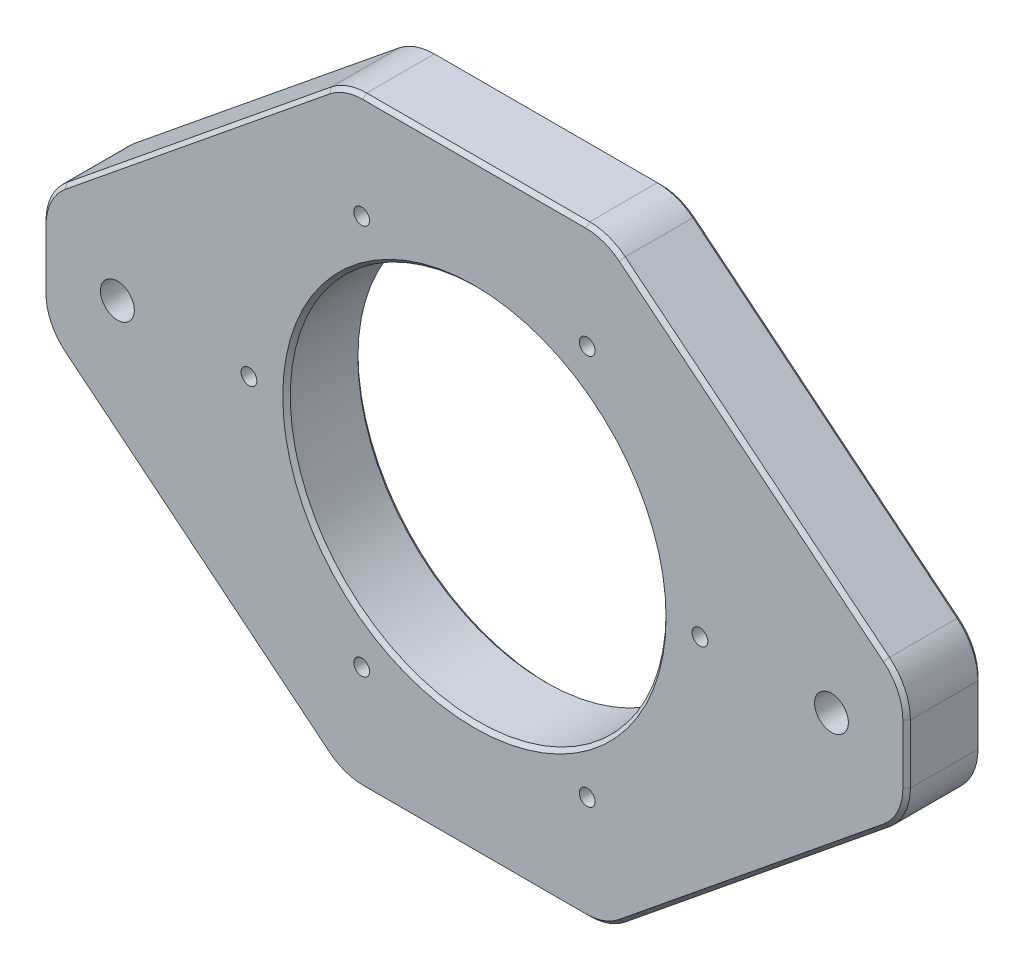
SolidWorks part; units mm, degrees
material "P20"
ref_plane "Front Plane" through (0, 0, 0) normal (0, 0, 1) x (1, 0, 0)
ref_plane "Top Plane" through (0, 0, 0) normal (0, 1, 0) x (1, 0, 0)
ref_plane "Right Plane" through (0, 0, 0) normal (1, 0, 0) x (0, 0, -1)
sketch "Sketch1" plane through (0, 0, 0) normal (0, 0, 1) x (1, 0, 0)
  line L1 (-115, -80) -> (115, -80)
  line L2 (-115, -80) -> (-115, 80)
  line L3 (-115, 80) -> (115, 80)
  line L4 (115, -80) -> (115, 80)
  line L5 (-115, -80) -> (115, 80) construction
  line L6 (-115, 80) -> (115, -80) construction
  circle A0 centre (0, 0) radius 115 construction
  point P0 (0, 0)
  dimension "D3" = 230
  dimension "D1" = 230
  dimension "D2" = 160
extrude "Boss-Extrude1" add sketch "Sketch1" along normal blind 20
sketch "Sketch4" plane through (0, 0, 20) normal (0, 0, 1) x (1, 0, 0)
  circle A0 centre (0, 0) radius 50
  dimension "D1" = 100
extrude "Cut-Extrude3" cut sketch "Sketch4" against normal blind 109
sketch "Sketch5" plane through (0, 0, 0) normal (0, 0, 1) x (1, 0, 0)
  line L0 (0, 0) -> (-95, 0) construction
  line L1 (0, 0) -> (95, 0) construction
  line L2 (0, 0) -> (0, 179.4506) construction
  circle A0 centre (-95, 0) radius 10.25
  circle A1 centre (95, 0) radius 10.25
  dimension "D1" = 20.5
  dimension "D2" = 190
extrude "Cut-Extrude4" cut sketch "Sketch5" along normal blind 6
hole_wizard "M8 Clearance Hole1" positions "Sketch6" profile "Sketch8" hole size "M8" standard "GB" end condition through all
sketch "Sketch6" plane through (0, 0, 20) normal (0, 0, 1) x (1, 0, 0)
  point P0 (-95, 0)
  point P2 (95, 0)
sketch "Sketch8" plane through (-95, 0, 20) normal (1, 0, 0) x (0, -1, 0)
  line L0 (0, 0) -> (0, 20)
  line L1 (0, 20) -> (4.5, 20)
  line L2 (4.5, 20) -> (4.5, 0)
  line L5 (4.5, 0) -> (0, 0)
  line L11 (0, -6.35) -> (0, 107.95) construction
  dimension "通孔孔直径" = 9
  dimension "通孔孔深度" = 20
chamfer "Chamfer2" distance 1 angle 45 2 edges at (50, 0, 20) (-50, 0, 0)
sketch "Sketch10" plane through (0, 0, 20) normal (0, 0, 1) x (1, 0, 0)
  line L0 (-115, 80) -> (-35, 80)
  line L1 (115, 80) -> (-115, 80) construction
  line L2 (-35, 80) -> (-115, 15)
  line L3 (-115, 80) -> (-115, -80) construction
  line L4 (-115, 15) -> (-115, 80)
  line L5 (35, 80) -> (115, 80)
  line L6 (115, 80) -> (115, 15)
  line L7 (115, -80) -> (115, 80) construction
  line L8 (115, 15) -> (35, 80)
  line L9 (-115, -15) -> (-35, -80)
  line L10 (-115, -80) -> (115, -80) construction
  line L11 (-35, -80) -> (-115, -80)
  line L12 (-115, -80) -> (-115, -15)
  line L13 (35, -80) -> (115, -80)
  line L14 (115, -80) -> (115, -15)
  line L15 (115, -15) -> (35, -80)
  line L16 (0, 80) -> (0, -80) construction
  line L17 (-115, 0) -> (115, 0) construction
  dimension "D1" = 80
  dimension "D2" = 65
extrude "Cut-Extrude6" cut sketch "Sketch10" against normal blind 214
fillet "Fillet1" radius 15 8 edges at (-115, 15, 10) (-35, 80, 10) (35, 80, 10) (115, 15, 10) (115, -15, 10) (35, -80, 10) (-35, -80, 10) (-115, -15, 10)
chamfer "Chamfer3" distance 1 angle 45 32 edges at (115, 0, 0) (113.5441, 14.307, 0) (113.5441, -14.307, 0) (74.2961, 48.0719, 0) (74.2961, -48.0719, 0) (34.6931, 79.1355, 0) (34.6931, -79.1355, 0) (0, 80, 0) (0, -80, 0) (-34.6931, 79.1355, 0) (-34.6931, -79.1355, 0) (-74.2961, 48.0719, 0) (-74.2961, -48.0719, 0) (-113.5441, 14.307, 0) (-113.5441, -14.307, 0) (-115, 0, 0) (74.2961, -48.0719, 20) (34.6931, -79.1355, 20) (113.5441, -14.307, 20) (0, -80, 20) (115, 0, 20) (-34.6931, -79.1355, 20) (113.5441, 14.307, 20) (-74.2961, -48.0719, 20) (74.2961, 48.0719, 20) (-113.5441, -14.307, 20) (34.6931, 79.1355, 20) (-115, 0, 20) (0, 80, 20) (-113.5441, 14.307, 20) (-34.6931, 79.1355, 20) (-74.2961, 48.0719, 20)
chamfer "Chamfer4" distance 1 angle 45 2 edges at (105.25, 0, 0) (-84.75, 0, 0)
hole_wizard "M5 Tapped Hole1" positions "Sketch11" profile "Sketch12" tap size "M5" standard "GB" end condition through all
sketch "Sketch11" plane through (0, 0, 20) normal (0, 0, 1) x (1, 0, 0)
  point P0 (-30, 51.9615)
  point P3 (-60, 0)
  point P6 (-30, -51.9615)
  point P9 (30, -51.9615)
  point P12 (60, 0)
  point P15 (30, 51.9615)
sketch "Sketch12" plane through (-30, 51.9615, 20) normal (1, 0, 0) x (0, -1, 0)
  line L0 (0, 0) -> (0, 20)
  line L1 (0, 20) -> (2.1, 20)
  line L2 (2.1, 20) -> (2.1, 0)
  line L5 (2.1, 0) -> (0, 0)
  line L11 (0, -6.35) -> (0, 107.95) construction
  dimension "通孔螺纹孔钻头直径" = 4.2
  dimension "通孔螺纹孔钻头深度" = 20
cosmetic thread "Cosmetic thread 1" parameters "D2"=5
cosmetic thread "Cosmetic thread 2" parameters "D2"=5
cosmetic thread "Cosmetic thread 3" parameters "D2"=5
cosmetic thread "Cosmetic thread 4" parameters "D2"=5
cosmetic thread "Cosmetic thread 5" parameters "D2"=5
cosmetic thread "Cosmetic thread 6" parameters "D2"=5
